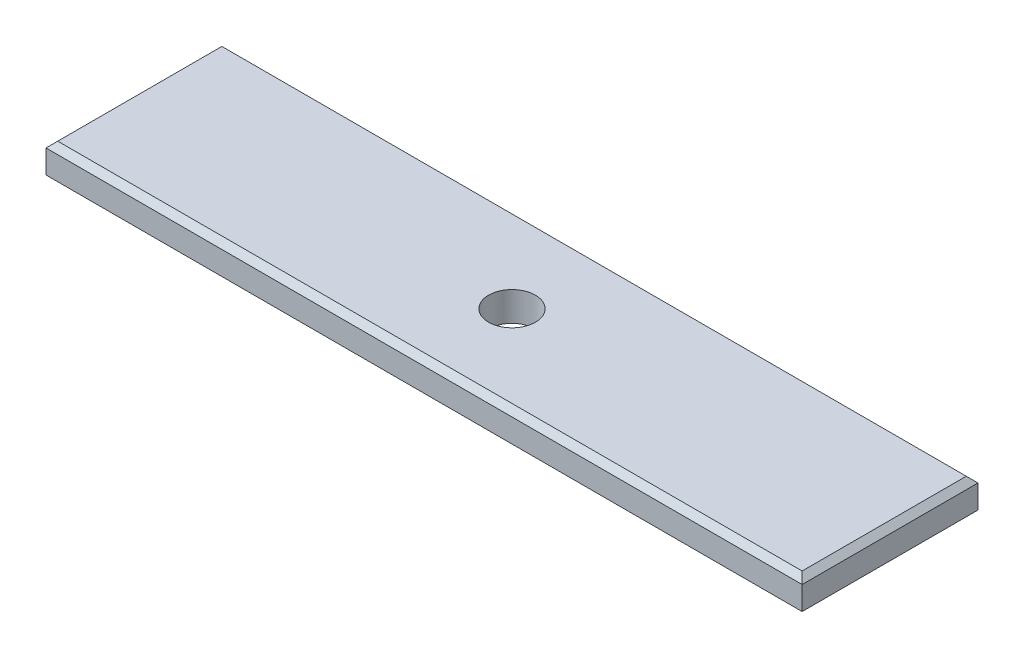
from build123d import *

# Parameters (mm, degrees)
SKETCH1_W           = 129
SKETCH1_H           = 30
BOSS_EXTRUDE1_DEPTH = 5
CUT_EXTRUDE1_REACH  = 68.41
SKETCH3_R           = 4
CHAMFER1_SIZE       = 1


with BuildPart() as part:
    # Sketch1 → Boss-Extrude1 (new body)
    with BuildSketch(Plane(origin=(0, 0, 0), x_dir=(1, 0, 0), z_dir=(0, 1, 0))):
        Rectangle(SKETCH1_W, SKETCH1_H)
    extrude(amount=BOSS_EXTRUDE1_DEPTH)

    # Sketch3 → Cut-Extrude1 (cut, up to next)
    with BuildSketch(Plane(origin=(0, 5, 0), x_dir=(1, 0, 0), z_dir=(0, 1, 0)), mode=Mode.PRIVATE) as cut_extrude1_sk1:
        with Locations(Location((0, 0, 0), (0, 0, 270))):
            Circle(SKETCH3_R)
    cut_extrude1_tool1 = extrude(cut_extrude1_sk1.sketch, amount=-CUT_EXTRUDE1_REACH, mode=Mode.PRIVATE) & part.part
    add(cut_extrude1_tool1.solids().sort_by_distance((0, 5, 0))[0], mode=Mode.SUBTRACT)

    # Chamfer1
    chamfer1_edges = [part.edges().sort_by_distance(p)[0] for p in [
        (-64.5, 5, 0),
        (0, 5, 15),
        (64.5, 5, 0),
        (0, 5, -15),
    ]]
    chamfer(chamfer1_edges, length=CHAMFER1_SIZE)


solid = part.part
